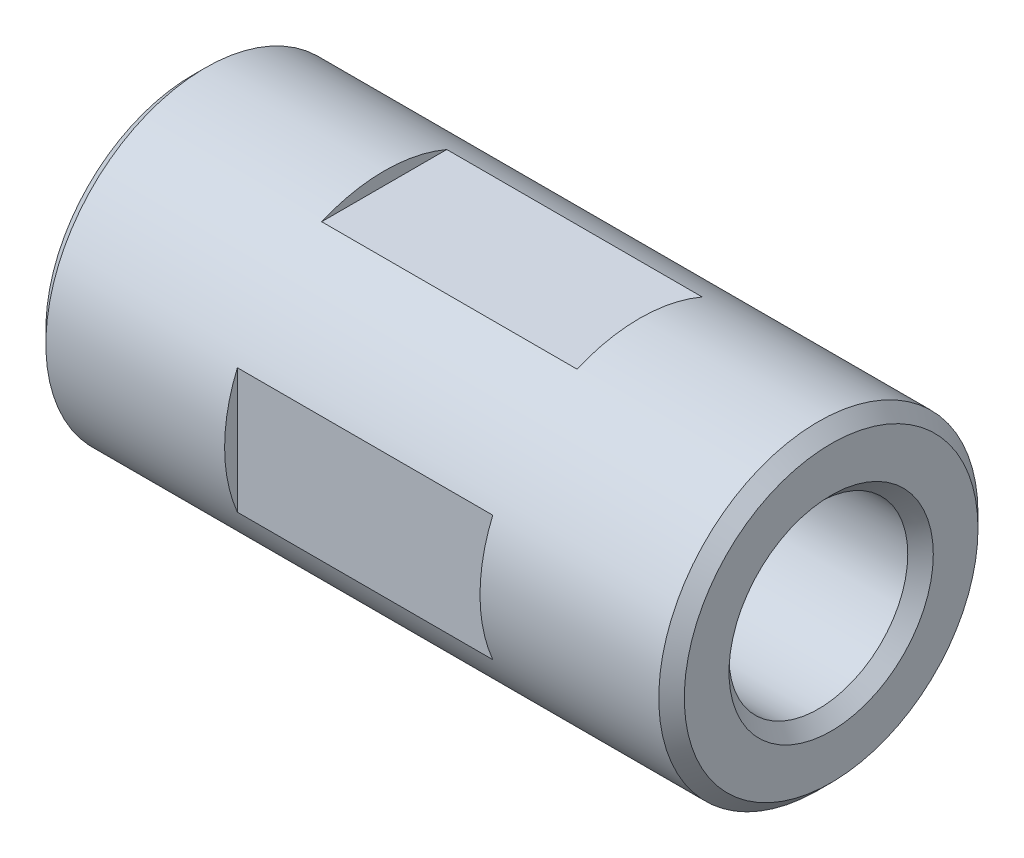
from build123d import *

# Parameters (mm, degrees)
SKETCH_1_R           = 12.5
EXTRUDE_1_DEPTH      = 25
HOLE_WIZARD_M16_1_D  = 14
SKETCH_4_OUTSIDE_W   = 39.248
SKETCH_4_OUTSIDE_H   = 39.248
SKETCH_4_OUTSIDE_W_2 = 23
SKETCH_4_OUTSIDE_H_2 = 23
CUT_EXTRUDE_1_DEPTH  = 10
CHAMFER_1_SIZE       = 1


with BuildPart() as part:
    # 草图1 → 凸台-拉伸1 (new, symmetric)
    with BuildSketch(Plane(origin=(0, 0, 0), x_dir=(0, 0, -1), z_dir=(1, 0, 0))):
        Circle(SKETCH_1_R)
    extrude(amount=EXTRUDE_1_DEPTH, both=True)

    # M16 螺纹孔1 (through all)
    with Locations(Plane(origin=(25, 0, 0), x_dir=(0, 0, -1), z_dir=(1, 0, 0))):
        with Locations((0, 0)):
            Hole(HOLE_WIZARD_M16_1_D / 2)

    # 草图4 outside → 切除-拉伸1 (cut, symmetric)
    with BuildSketch(Plane(origin=(0, 0, 0), x_dir=(0, 0, -1), z_dir=(1, 0, 0))):
        Rectangle(SKETCH_4_OUTSIDE_W, SKETCH_4_OUTSIDE_H)
        Rectangle(SKETCH_4_OUTSIDE_W_2, SKETCH_4_OUTSIDE_H_2, mode=Mode.SUBTRACT)
    extrude(amount=CUT_EXTRUDE_1_DEPTH, both=True, mode=Mode.SUBTRACT)

    # 倒角1
    chamfer_1_edges = [part.edges().sort_by_distance(p)[0] for p in [
        (-25, 0, 12.5),
        (25, 0, 12.5),
        (25, 0, -7),
        (-25, 0, -7),
    ]]
    chamfer(chamfer_1_edges, length=CHAMFER_1_SIZE)


solid = part.part
